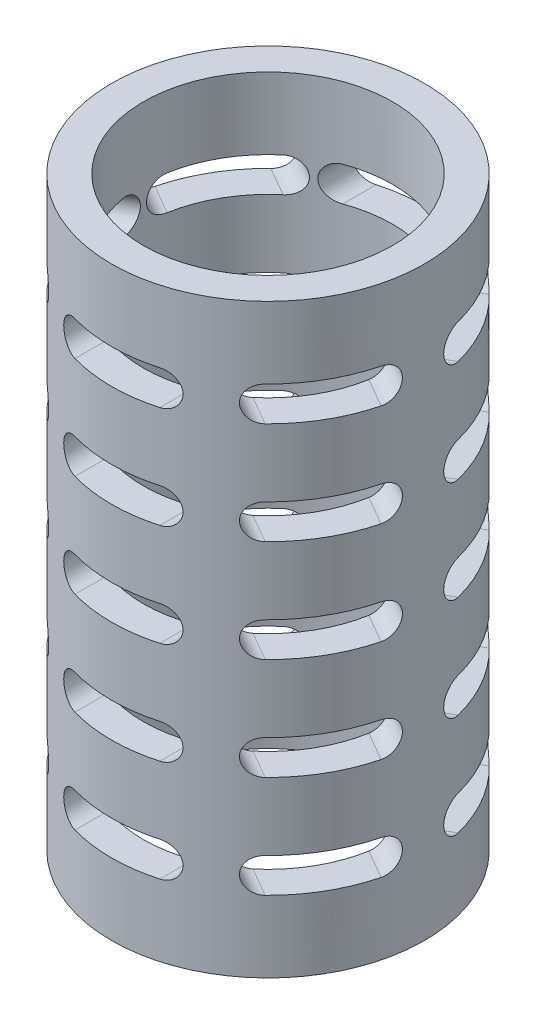
from build123d import *

# Parameters (mm, degrees)
SKETCH1_R               = 59
SKETCH1_R_2             = 47
BOSS_EXTRUDE1_DEPTH     = 221
CUT_EXTRUDE1_DEPTH      = 221
CIRPATTERN1_COUNT       = 6
LPATTERN1_COUNT         = 5
LPATTERN1_PITCH         = 38.5
LPATTERN1_COPY_1_DEPTH  = 221
LPATTERN1_COPY_2_DEPTH  = 221
LPATTERN1_COPY_3_DEPTH  = 221
LPATTERN1_COPY_4_DEPTH  = 221
LPATTERN1_COPY_5_DEPTH  = 221
LPATTERN1_COPY_6_DEPTH  = 221
LPATTERN1_COPY_7_DEPTH  = 221
LPATTERN1_COPY_8_DEPTH  = 221
LPATTERN1_COPY_9_DEPTH  = 221
LPATTERN1_COPY_10_DEPTH = 221
LPATTERN1_COPY_11_DEPTH = 221
LPATTERN1_COPY_12_DEPTH = 221
LPATTERN1_COPY_13_DEPTH = 221
LPATTERN1_COPY_14_DEPTH = 221
LPATTERN1_COPY_15_DEPTH = 221
LPATTERN1_COPY_16_DEPTH = 221
LPATTERN1_COPY_17_DEPTH = 221
LPATTERN1_COPY_18_DEPTH = 221
LPATTERN1_COPY_19_DEPTH = 221
LPATTERN1_COPY_20_DEPTH = 221


with BuildPart() as part:
    # Sketch1 → Boss-Extrude1 (new body)
    with BuildSketch(Plane(origin=(0, 0, 0), x_dir=(1, 0, 0), z_dir=(0, 1, 0))):
        with Locations(Location((0, 0, 0), (0, 0, 270))):
            Circle(SKETCH1_R)
        with Locations(Location((0, 0, 0), (0, 0, 270))):
            Circle(SKETCH1_R_2, mode=Mode.SUBTRACT)
    extrude(amount=BOSS_EXTRUDE1_DEPTH)

    # Sketch2 → Cut-Extrude1 (cut)
    with BuildSketch(Plane.XY):
        with BuildLine():
            Line((-16, 194), (16, 194))
            ThreePointArc((16, 194), (22.5, 187.5), (16, 181))
            Line((16, 181), (-16, 181))
            ThreePointArc((-16, 181), (-22.5, 187.5), (-16, 194))
        make_face()
    cut_extrude1 = extrude(amount=-CUT_EXTRUDE1_DEPTH, mode=Mode.SUBTRACT)

    # CirPattern1: Cut-Extrude1 ×6 about axis
    cirpattern1_axis = Axis((0, 221, 0), (0, 1, 0))
    for i in range(1, CIRPATTERN1_COUNT):
        add(cut_extrude1.rotate(cirpattern1_axis, i * 360 / CIRPATTERN1_COUNT), mode=Mode.SUBTRACT)

    # LPattern1: Cut-Extrude1 ×5
    with Locations(*[(0, -i * LPATTERN1_PITCH, 0) for i in range(1, LPATTERN1_COUNT)]):
        add(cut_extrude1, mode=Mode.SUBTRACT)

    # LPattern1 copy 1 sketch → LPattern1 copy 1 (cut)
    with BuildSketch(Plane(origin=(0, -38.5, 0), x_dir=(0.5000000000000001, 0, -0.8660254037844386), z_dir=(0.8660254037844386, 0, 0.5000000000000001))):
        with BuildLine():
            Line((-16, 194), (16, 194))
            ThreePointArc((16, 194), (22.5, 187.5), (16, 181))
            Line((16, 181), (-16, 181))
            ThreePointArc((-16, 181), (-22.5, 187.5), (-16, 194))
        make_face()
    extrude(amount=-LPATTERN1_COPY_1_DEPTH, mode=Mode.SUBTRACT)

    # LPattern1 copy 2 sketch → LPattern1 copy 2 (cut)
    with BuildSketch(Plane(origin=(0, -77, 0), x_dir=(0.5000000000000001, 0, -0.8660254037844386), z_dir=(0.8660254037844386, 0, 0.5000000000000001))):
        with BuildLine():
            Line((-16, 194), (16, 194))
            ThreePointArc((16, 194), (22.5, 187.5), (16, 181))
            Line((16, 181), (-16, 181))
            ThreePointArc((-16, 181), (-22.5, 187.5), (-16, 194))
        make_face()
    extrude(amount=-LPATTERN1_COPY_2_DEPTH, mode=Mode.SUBTRACT)

    # LPattern1 copy 3 sketch → LPattern1 copy 3 (cut)
    with BuildSketch(Plane(origin=(0, -115.5, 0), x_dir=(0.5000000000000001, 0, -0.8660254037844386), z_dir=(0.8660254037844386, 0, 0.5000000000000001))):
        with BuildLine():
            Line((-16, 194), (16, 194))
            ThreePointArc((16, 194), (22.5, 187.5), (16, 181))
            Line((16, 181), (-16, 181))
            ThreePointArc((-16, 181), (-22.5, 187.5), (-16, 194))
        make_face()
    extrude(amount=-LPATTERN1_COPY_3_DEPTH, mode=Mode.SUBTRACT)

    # LPattern1 copy 4 sketch → LPattern1 copy 4 (cut)
    with BuildSketch(Plane(origin=(0, -154, 0), x_dir=(0.5000000000000001, 0, -0.8660254037844386), z_dir=(0.8660254037844386, 0, 0.5000000000000001))):
        with BuildLine():
            Line((-16, 194), (16, 194))
            ThreePointArc((16, 194), (22.5, 187.5), (16, 181))
            Line((16, 181), (-16, 181))
            ThreePointArc((-16, 181), (-22.5, 187.5), (-16, 194))
        make_face()
    extrude(amount=-LPATTERN1_COPY_4_DEPTH, mode=Mode.SUBTRACT)

    # LPattern1 copy 5 sketch → LPattern1 copy 5 (cut)
    with BuildSketch(Plane(origin=(0, -38.5, 0), x_dir=(-0.4999999999999998, 0, -0.8660254037844387), z_dir=(0.8660254037844387, 0, -0.4999999999999998))):
        with BuildLine():
            Line((-16, 194), (16, 194))
            ThreePointArc((16, 194), (22.5, 187.5), (16, 181))
            Line((16, 181), (-16, 181))
            ThreePointArc((-16, 181), (-22.5, 187.5), (-16, 194))
        make_face()
    extrude(amount=-LPATTERN1_COPY_5_DEPTH, mode=Mode.SUBTRACT)

    # LPattern1 copy 6 sketch → LPattern1 copy 6 (cut)
    with BuildSketch(Plane(origin=(0, -77, 0), x_dir=(-0.4999999999999998, 0, -0.8660254037844387), z_dir=(0.8660254037844387, 0, -0.4999999999999998))):
        with BuildLine():
            Line((-16, 194), (16, 194))
            ThreePointArc((16, 194), (22.5, 187.5), (16, 181))
            Line((16, 181), (-16, 181))
            ThreePointArc((-16, 181), (-22.5, 187.5), (-16, 194))
        make_face()
    extrude(amount=-LPATTERN1_COPY_6_DEPTH, mode=Mode.SUBTRACT)

    # LPattern1 copy 7 sketch → LPattern1 copy 7 (cut)
    with BuildSketch(Plane(origin=(0, -115.5, 0), x_dir=(-0.4999999999999998, 0, -0.8660254037844387), z_dir=(0.8660254037844387, 0, -0.4999999999999998))):
        with BuildLine():
            Line((-16, 194), (16, 194))
            ThreePointArc((16, 194), (22.5, 187.5), (16, 181))
            Line((16, 181), (-16, 181))
            ThreePointArc((-16, 181), (-22.5, 187.5), (-16, 194))
        make_face()
    extrude(amount=-LPATTERN1_COPY_7_DEPTH, mode=Mode.SUBTRACT)

    # LPattern1 copy 8 sketch → LPattern1 copy 8 (cut)
    with BuildSketch(Plane(origin=(0, -154, 0), x_dir=(-0.4999999999999998, 0, -0.8660254037844387), z_dir=(0.8660254037844387, 0, -0.4999999999999998))):
        with BuildLine():
            Line((-16, 194), (16, 194))
            ThreePointArc((16, 194), (22.5, 187.5), (16, 181))
            Line((16, 181), (-16, 181))
            ThreePointArc((-16, 181), (-22.5, 187.5), (-16, 194))
        make_face()
    extrude(amount=-LPATTERN1_COPY_8_DEPTH, mode=Mode.SUBTRACT)

    # LPattern1 copy 9 sketch → LPattern1 copy 9 (cut)
    with BuildSketch(Plane(origin=(0, -38.5, 0), x_dir=(-1, 0, 0), z_dir=(0, 0, -1))):
        with BuildLine():
            Line((-16, 194), (16, 194))
            ThreePointArc((16, 194), (22.5, 187.5), (16, 181))
            Line((16, 181), (-16, 181))
            ThreePointArc((-16, 181), (-22.5, 187.5), (-16, 194))
        make_face()
    extrude(amount=-LPATTERN1_COPY_9_DEPTH, mode=Mode.SUBTRACT)

    # LPattern1 copy 10 sketch → LPattern1 copy 10 (cut)
    with BuildSketch(Plane(origin=(0, -77, 0), x_dir=(-1, 0, 0), z_dir=(0, 0, -1))):
        with BuildLine():
            Line((-16, 194), (16, 194))
            ThreePointArc((16, 194), (22.5, 187.5), (16, 181))
            Line((16, 181), (-16, 181))
            ThreePointArc((-16, 181), (-22.5, 187.5), (-16, 194))
        make_face()
    extrude(amount=-LPATTERN1_COPY_10_DEPTH, mode=Mode.SUBTRACT)

    # LPattern1 copy 11 sketch → LPattern1 copy 11 (cut)
    with BuildSketch(Plane(origin=(0, -115.5, 0), x_dir=(-1, 0, 0), z_dir=(0, 0, -1))):
        with BuildLine():
            Line((-16, 194), (16, 194))
            ThreePointArc((16, 194), (22.5, 187.5), (16, 181))
            Line((16, 181), (-16, 181))
            ThreePointArc((-16, 181), (-22.5, 187.5), (-16, 194))
        make_face()
    extrude(amount=-LPATTERN1_COPY_11_DEPTH, mode=Mode.SUBTRACT)

    # LPattern1 copy 12 sketch → LPattern1 copy 12 (cut)
    with BuildSketch(Plane(origin=(0, -154, 0), x_dir=(-1, 0, 0), z_dir=(0, 0, -1))):
        with BuildLine():
            Line((-16, 194), (16, 194))
            ThreePointArc((16, 194), (22.5, 187.5), (16, 181))
            Line((16, 181), (-16, 181))
            ThreePointArc((-16, 181), (-22.5, 187.5), (-16, 194))
        make_face()
    extrude(amount=-LPATTERN1_COPY_12_DEPTH, mode=Mode.SUBTRACT)

    # LPattern1 copy 13 sketch → LPattern1 copy 13 (cut)
    with BuildSketch(Plane(origin=(0, -38.5, 0), x_dir=(-0.5000000000000004, 0, 0.8660254037844384), z_dir=(-0.8660254037844384, 0, -0.5000000000000004))):
        with BuildLine():
            Line((-16, 194), (16, 194))
            ThreePointArc((16, 194), (22.5, 187.5), (16, 181))
            Line((16, 181), (-16, 181))
            ThreePointArc((-16, 181), (-22.5, 187.5), (-16, 194))
        make_face()
    extrude(amount=-LPATTERN1_COPY_13_DEPTH, mode=Mode.SUBTRACT)

    # LPattern1 copy 14 sketch → LPattern1 copy 14 (cut)
    with BuildSketch(Plane(origin=(0, -77, 0), x_dir=(-0.5000000000000004, 0, 0.8660254037844384), z_dir=(-0.8660254037844384, 0, -0.5000000000000004))):
        with BuildLine():
            Line((-16, 194), (16, 194))
            ThreePointArc((16, 194), (22.5, 187.5), (16, 181))
            Line((16, 181), (-16, 181))
            ThreePointArc((-16, 181), (-22.5, 187.5), (-16, 194))
        make_face()
    extrude(amount=-LPATTERN1_COPY_14_DEPTH, mode=Mode.SUBTRACT)

    # LPattern1 copy 15 sketch → LPattern1 copy 15 (cut)
    with BuildSketch(Plane(origin=(0, -115.5, 0), x_dir=(-0.5000000000000004, 0, 0.8660254037844384), z_dir=(-0.8660254037844384, 0, -0.5000000000000004))):
        with BuildLine():
            Line((-16, 194), (16, 194))
            ThreePointArc((16, 194), (22.5, 187.5), (16, 181))
            Line((16, 181), (-16, 181))
            ThreePointArc((-16, 181), (-22.5, 187.5), (-16, 194))
        make_face()
    extrude(amount=-LPATTERN1_COPY_15_DEPTH, mode=Mode.SUBTRACT)

    # LPattern1 copy 16 sketch → LPattern1 copy 16 (cut)
    with BuildSketch(Plane(origin=(0, -154, 0), x_dir=(-0.5000000000000004, 0, 0.8660254037844384), z_dir=(-0.8660254037844384, 0, -0.5000000000000004))):
        with BuildLine():
            Line((-16, 194), (16, 194))
            ThreePointArc((16, 194), (22.5, 187.5), (16, 181))
            Line((16, 181), (-16, 181))
            ThreePointArc((-16, 181), (-22.5, 187.5), (-16, 194))
        make_face()
    extrude(amount=-LPATTERN1_COPY_16_DEPTH, mode=Mode.SUBTRACT)

    # LPattern1 copy 17 sketch → LPattern1 copy 17 (cut)
    with BuildSketch(Plane(origin=(0, -38.5, 0), x_dir=(0.5000000000000001, 0, 0.8660254037844386), z_dir=(-0.8660254037844386, 0, 0.5000000000000001))):
        with BuildLine():
            Line((-16, 194), (16, 194))
            ThreePointArc((16, 194), (22.5, 187.5), (16, 181))
            Line((16, 181), (-16, 181))
            ThreePointArc((-16, 181), (-22.5, 187.5), (-16, 194))
        make_face()
    extrude(amount=-LPATTERN1_COPY_17_DEPTH, mode=Mode.SUBTRACT)

    # LPattern1 copy 18 sketch → LPattern1 copy 18 (cut)
    with BuildSketch(Plane(origin=(0, -77, 0), x_dir=(0.5000000000000001, 0, 0.8660254037844386), z_dir=(-0.8660254037844386, 0, 0.5000000000000001))):
        with BuildLine():
            Line((-16, 194), (16, 194))
            ThreePointArc((16, 194), (22.5, 187.5), (16, 181))
            Line((16, 181), (-16, 181))
            ThreePointArc((-16, 181), (-22.5, 187.5), (-16, 194))
        make_face()
    extrude(amount=-LPATTERN1_COPY_18_DEPTH, mode=Mode.SUBTRACT)

    # LPattern1 copy 19 sketch → LPattern1 copy 19 (cut)
    with BuildSketch(Plane(origin=(0, -115.5, 0), x_dir=(0.5000000000000001, 0, 0.8660254037844386), z_dir=(-0.8660254037844386, 0, 0.5000000000000001))):
        with BuildLine():
            Line((-16, 194), (16, 194))
            ThreePointArc((16, 194), (22.5, 187.5), (16, 181))
            Line((16, 181), (-16, 181))
            ThreePointArc((-16, 181), (-22.5, 187.5), (-16, 194))
        make_face()
    extrude(amount=-LPATTERN1_COPY_19_DEPTH, mode=Mode.SUBTRACT)

    # LPattern1 copy 20 sketch → LPattern1 copy 20 (cut)
    with BuildSketch(Plane(origin=(0, -154, 0), x_dir=(0.5000000000000001, 0, 0.8660254037844386), z_dir=(-0.8660254037844386, 0, 0.5000000000000001))):
        with BuildLine():
            Line((-16, 194), (16, 194))
            ThreePointArc((16, 194), (22.5, 187.5), (16, 181))
            Line((16, 181), (-16, 181))
            ThreePointArc((-16, 181), (-22.5, 187.5), (-16, 194))
        make_face()
    extrude(amount=-LPATTERN1_COPY_20_DEPTH, mode=Mode.SUBTRACT)


solid = part.part
